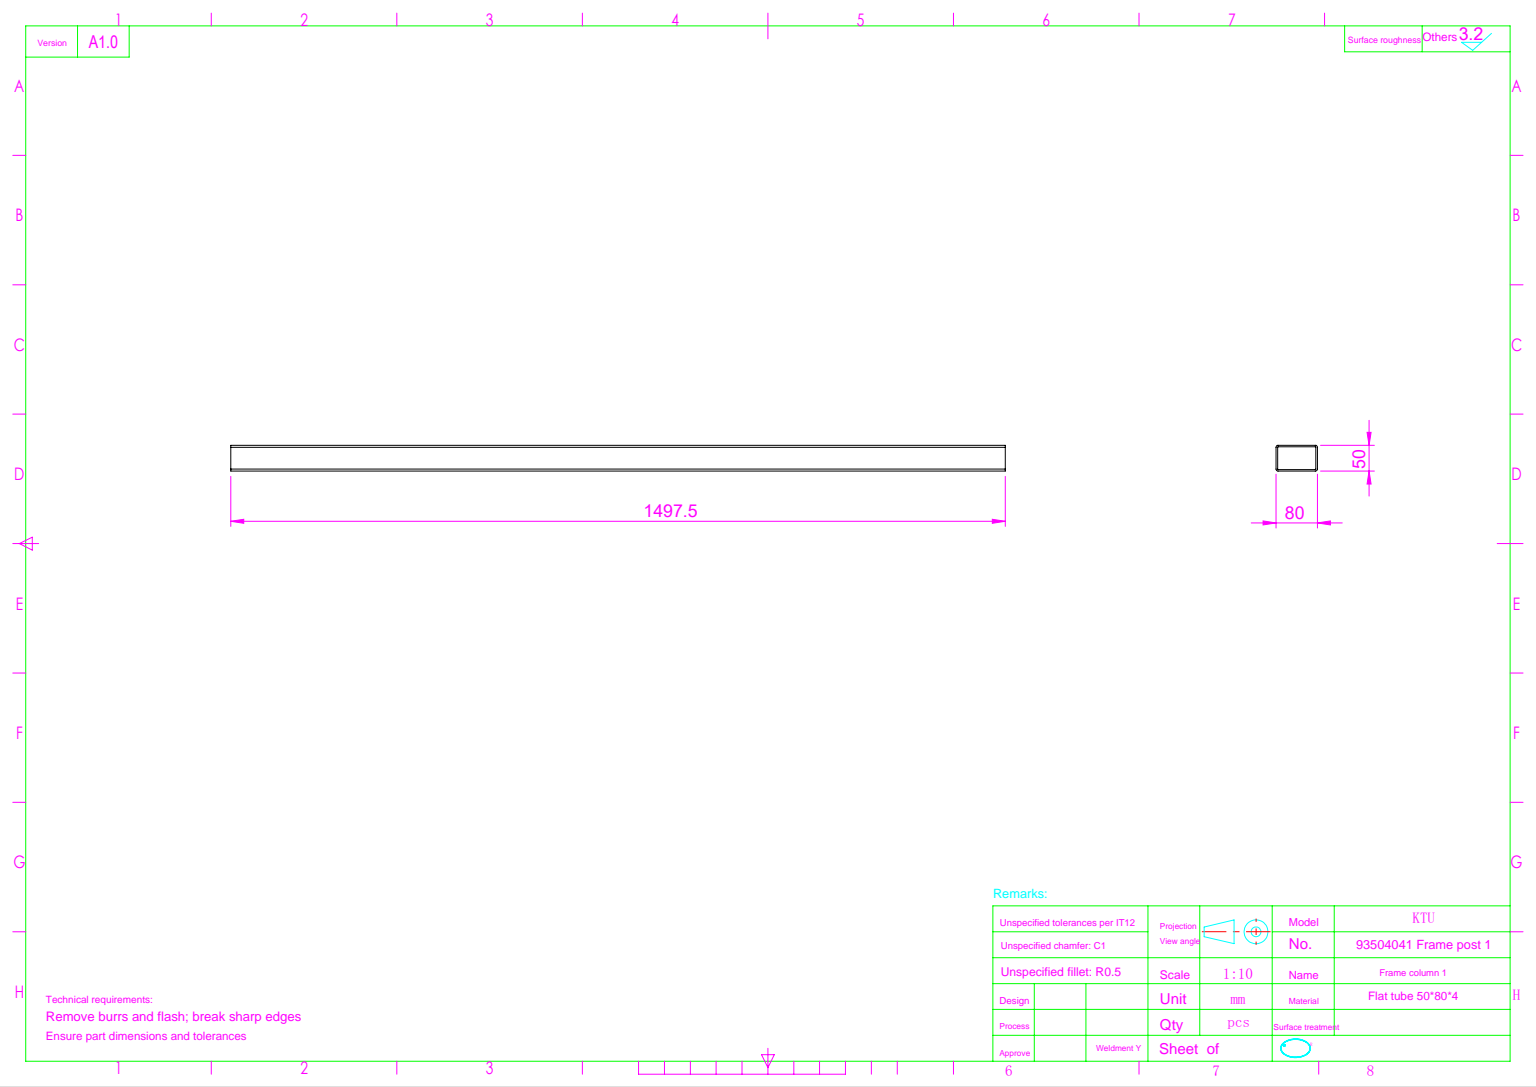
SolidWorks part; units mm, degrees
ref_plane "前视基准面" through (0, 0, 0) normal (0, 0, 1) x (1, 0, 0)
ref_plane "上视基准面" through (0, 0, 0) normal (0, 1, 0) x (1, 0, 0)
ref_plane "右视基准面" through (0, 0, 0) normal (1, 0, 0) x (0, 0, -1)
sketch "草图1" plane through (0, 0, 0) normal (0, 0, 1) x (1, 0, 0)
  line L1 (-36, 25) -> (36, 25)
  line L2 (-40, 21) -> (-40, -21)
  line L3 (-36, -25) -> (36, -25)
  line L4 (40, 21) -> (40, -21)
  line L5 (-40, 25) -> (40, -25) construction
  line L6 (-40, -25) -> (40, 25) construction
  arc A0 (36, -25) -> (40, -21) centre (36, -21) ccw
  arc A1 (-40, -21) -> (-36, -25) centre (-36, -21) ccw
  arc A2 (36, 25) -> (40, 21) centre (36, 21) cw
  arc A3 (-36, 25) -> (-40, 21) centre (-36, 21) ccw
  point P0 (0, 0)
  dimension "D3" = 4
  dimension "D1" = 50
  dimension "D2" = 80
extrude "拉伸-薄壁1" add sketch "草图1" along normal mid plane 1497.5 thin
